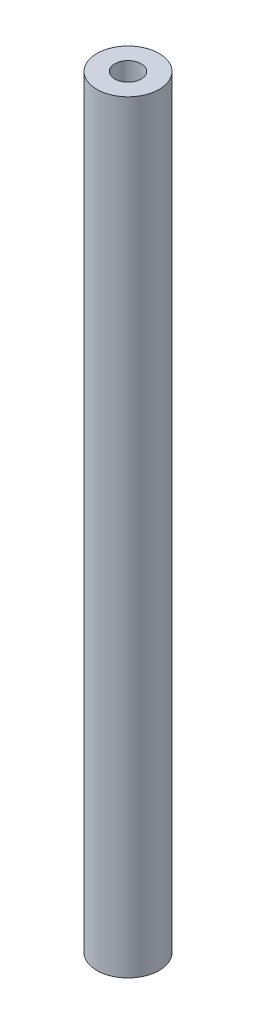
SolidWorks part; units mm, degrees
material "6061-T6 (SS)"
ref_plane "前视基准面" through (0, 0, 0) normal (0, 0, 1) x (1, 0, 0)
ref_plane "上视基准面" through (0, 0, 0) normal (0, 1, 0) x (1, 0, 0)
ref_plane "右视基准面" through (0, 0, 0) normal (1, 0, 0) x (0, 0, -1)
other "Configuration Table"
sketch "草图1" plane through (0, 0, 0) normal (0, 0, 1) x (1, 0, 0)
  line L0 (0, 0) -> (0, 196)
  dimension "D1" = 196
revolve "旋转-薄壁1" add sketch "草图1" angle 360 about L0 wall 8
hole_wizard "M8 螺纹孔的螺纹孔钻头1" positions "草图4" profile "草图5" hole size "M8" standard "GB"
sketch "草图4" plane through (0, 0, 0) normal (0, -1, 0) x (-1, 0, 0)
  point P0 (0, 0)
  point P3 (0, 0)
sketch "草图5" plane through (0, 0, 0) normal (1, 0, 0) x (0, 0, -1)
  line L0 (0, 0) -> (0, 10.0429)
  line L1 (0, 10.0429) -> (3.4, 8)
  line L2 (3.4, 8) -> (3.4, 0)
  line L5 (3.4, 0) -> (0, 0)
  line L10 (0, 10.0429) -> (-3.4, 8) construction
  line L11 (0, -6.35) -> (0, 107.95) construction
  dimension "孔直径" = 6.8
  dimension "孔深度" = 8
  dimension "导头角度" = 118
hole_wizard "M8 螺纹孔的螺纹孔钻头2" positions "草图6" profile "草图7" hole size "M8" standard "GB"
sketch "草图6" plane through (0, 196, 0) normal (0, 1, 0) x (1, 0, 0)
  point P0 (0, 0)
sketch "草图7" plane through (0, 196, 0) normal (1, 0, 0) x (0, 0, 1)
  line L0 (0, 0) -> (0, 10.0429)
  line L1 (0, 10.0429) -> (3.4, 8)
  line L2 (3.4, 8) -> (3.4, 0)
  line L5 (3.4, 0) -> (0, 0)
  line L10 (0, 10.0429) -> (-3.4, 8) construction
  line L11 (0, -6.35) -> (0, 107.95) construction
  dimension "孔直径" = 6.8
  dimension "孔深度" = 8
  dimension "导头角度" = 118
